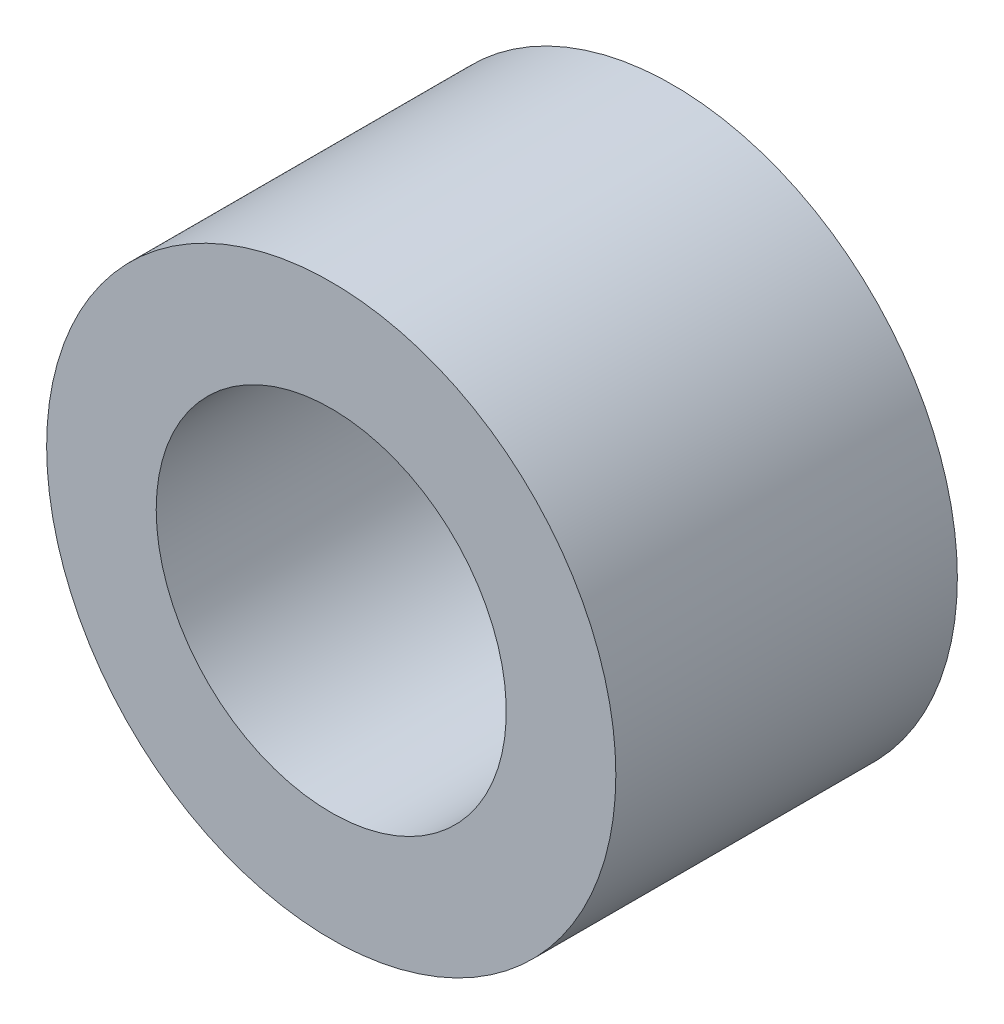
from build123d import *

# Parameters (mm, degrees)
SKETCH1_R           = 25
BOSS_EXTRUDE1_DEPTH = 30
G1_THREADED_HOLE1_D = 30.75


with BuildPart() as part:
    # Sketch1 → Boss-Extrude1 (new body)
    with BuildSketch(Plane.XY):
        Circle(SKETCH1_R)
    extrude(amount=BOSS_EXTRUDE1_DEPTH)

    # G1 Threaded hole1 (through all)
    with Locations(Plane(origin=(0, 0, 0), x_dir=(-1, 0, 0), z_dir=(0, 0, -1))):
        with Locations((0, 0)):
            Hole(G1_THREADED_HOLE1_D / 2)


solid = part.part
